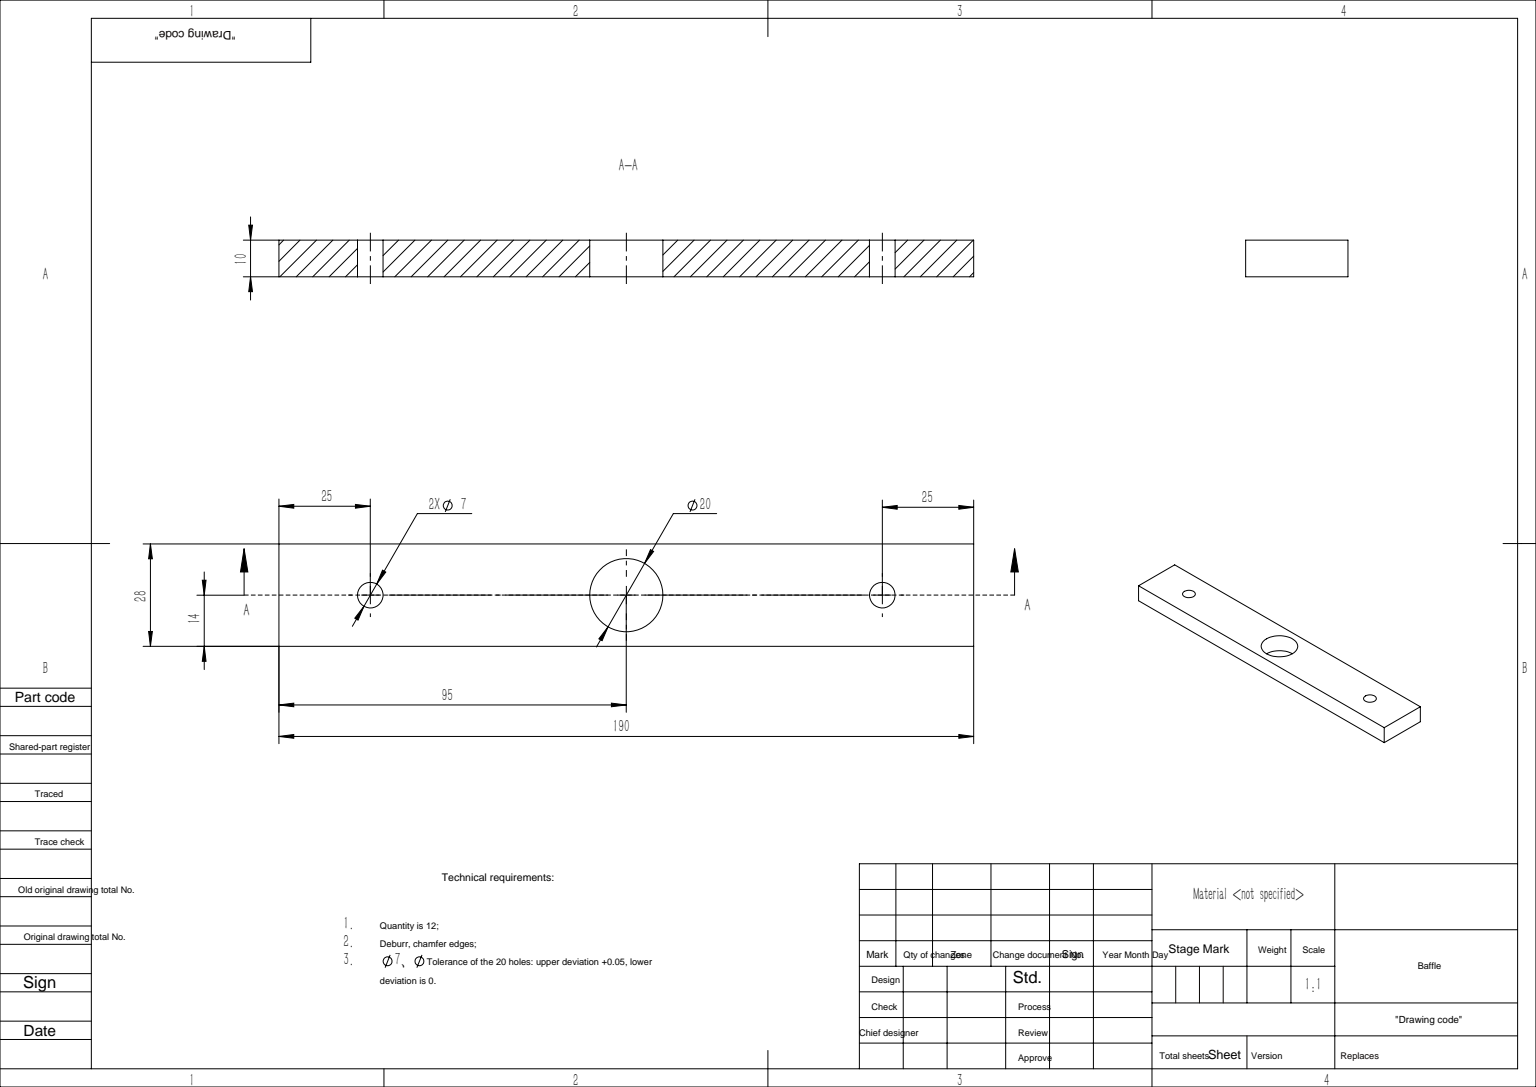
SolidWorks part; units mm, degrees
ref_plane "前视基准面" through (0, 0, 0) normal (0, 0, 1) x (1, 0, 0)
ref_plane "上视基准面" through (0, 0, 0) normal (0, 1, 0) x (1, 0, 0)
ref_plane "右视基准面" through (0, 0, 0) normal (1, 0, 0) x (0, 0, -1)
sketch "草图1" plane through (0, 1805.0003, 0) normal (0, 1, 0) x (1, 0, 0)
  line L0 (602.0857, 490.2759) -> (602.0857, 439.0183) construction
  line L1 (507.0857, 471) -> (507.0857, 459) construction
  line L2 (697.0857, 471) -> (697.0857, 459) construction
  line L3 (552.2729, 465) -> (754.3323, 465) construction
  line L4 (507.0857, 479) -> (697.0857, 479)
  line L5 (507.0857, 479) -> (507.0857, 451)
  line L6 (507.0857, 451) -> (697.0857, 451)
  line L7 (697.0857, 479) -> (697.0857, 451)
  line L8 (507.0857, 471) -> (557.0857, 471) construction
  line L9 (507.0857, 459) -> (557.0857, 459) construction
  dimension "D1" = 28
extrude "凸台-拉伸1" add sketch "草图1" along normal blind 10
sketch "草图2" plane through (0, 1815.0003, 0) normal (0, 1, 0) x (1, 0, 0)
  circle A0 centre (532.0857, 465) radius 3.5
  circle A1 centre (672.0857, 465) radius 3.5
  circle A2 centre (602.0857, 465) radius 10
  dimension "D1" = 7
  dimension "D2" = 20
extrude "切除-拉伸1" cut sketch "草图2" against normal through all
